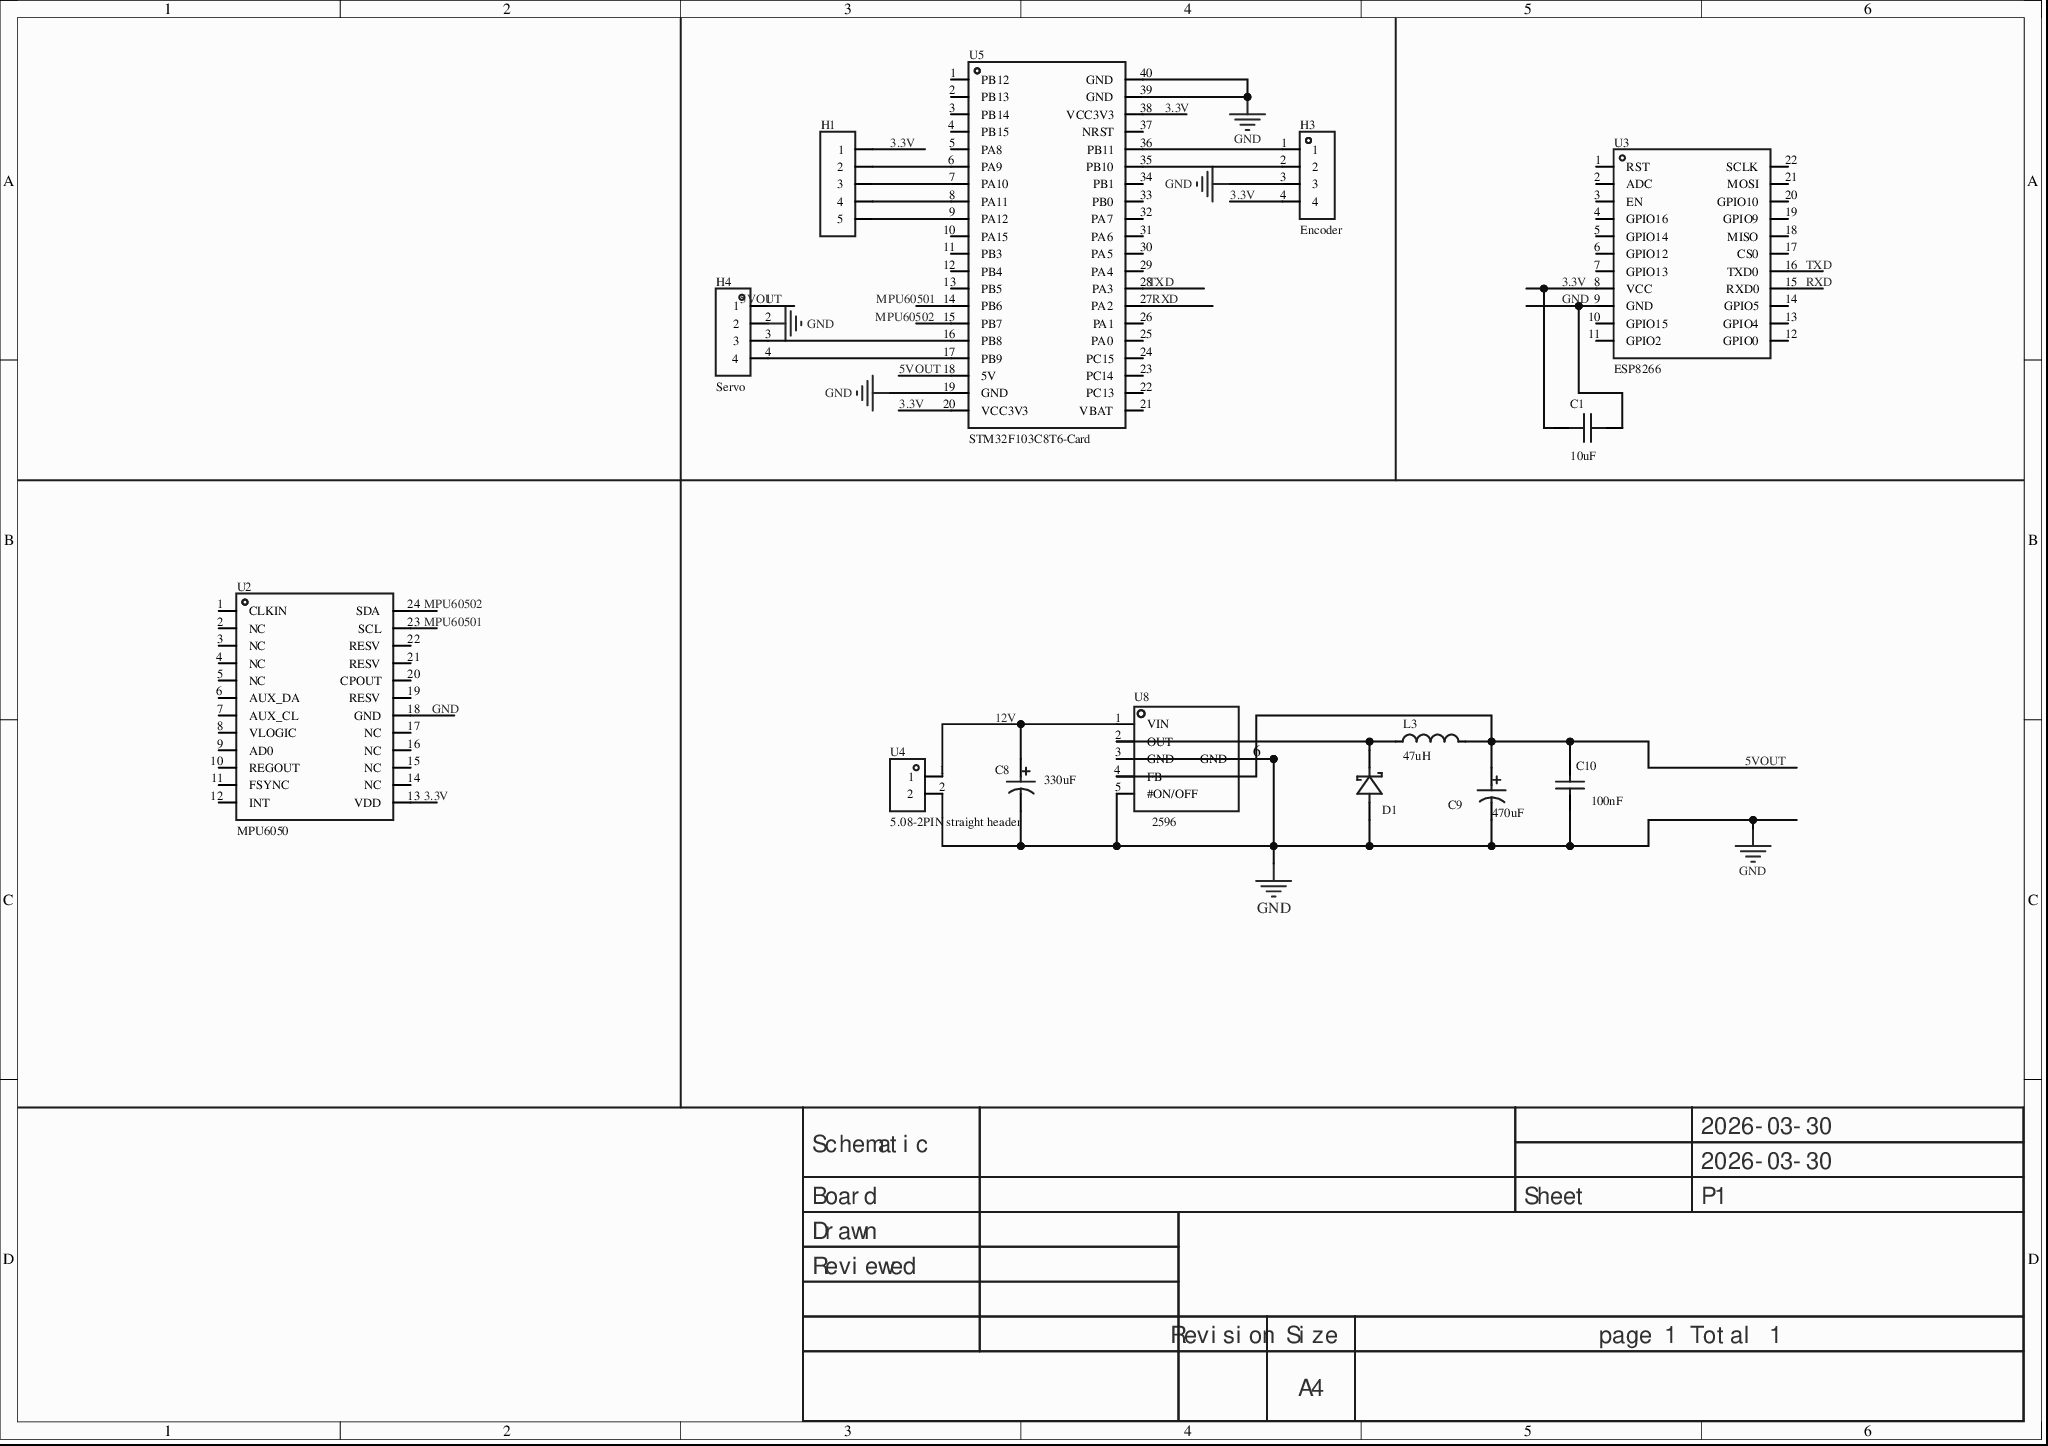
[diagram p0: MISC52071-3.schdoc]
# Altium project MISC52071-2.PrjPcb
1 sheet, 14 parts. Net scope: global (net labels, ports and power ports of the same name join across sheets).
Board file: MISC52071.pcbdoc

## Sheet MISC52071-3.schdoc
size 297 x 209 mm; Version: V1.0; @Project Name: MISC52071; @Update Date: 2026-03-30; @Create Date: 2026-03-30; @Board Name: MISC52071; @Create Time: 10:07:17; @Page Count: 1; @Page No: 1; @Schematic Name: MISC52071; @Update Time: 10:07:17; Size: A4

### Parts
C1  10uF  [C0603]
C8  value 330uF  [CAP-SMD_BD8.0-L8.3-W8.3-RD]
C9  value 470uF  [CAP-SMD_BD8.0-L8.3-W8.3-RD]
C10  value 100nF  [C0805]
D1  (no value)  [SMA_L4.3-W2.6-LS5.2-RD]
H1  (no value)  [HDR-TH_5P-P2.54-V-F]
H3  Encoder  [HDR-TH_4P-P2.54-V-M]
H4  Servo  [HDR-TH_4P-P2.54-V-M]
L3  value 47uH  [IND-SMD_L7.0-W6.6]
U2  MPU6050  [QFN-24_L4.0-W4.0-P0.50-BL]
U3  ESP8266  [WIFIM-SMD_ESP-12F-ESP8266MOD]
U4  5.08-2PIN straight header  [HDR-TH_2P-P5.08_C9900004333]
U5  STM32F103C8T6-Card  [CONN-TH_L53.3-W22.9_STM32F103C8T6-CARD]
U8  LM2596S-5.0  [TO-263-5_L10.2-W8.9-P1.70-BR]  (value not drawn)

### Nets
GND: C1.2 C8.2 C9.2 C10.2 D1.2(A) H3.3 H4.2 U2.18(GND) U3.9(GND) U4.2 U5.19(GND) U5.39(GND) U5.40(GND) U8.3(GND) U8.5(#ON/OFF) U8.6(GND)
3.3V: C1.1 H1.1 H3.4 U2.13(VDD) U3.8(VCC) U5.20(VCC3V3) U5.38(VCC3V3)
5VOUT: C9.1 C10.1 H4.1 L3.2 U5.18(5V) U8.4(FB)
12V: C8.1 U4.1 U8.1(VIN)
MPU60501: U2.23(SCL) U5.14(PB6)
MPU60502: U2.24(SDA) U5.15(PB7)
RXD: U3.15(RXD0) U5.27(PA2)
TXD: U3.16(TXD0) U5.28(PA3)
NetD1_1: D1.1(K) L3.1 U8.2(OUT)
NetH1_2: H1.2 U5.6(PA9)
NetH1_3: H1.3 U5.7(PA10)
NetH1_4: H1.4 U5.8(PA11)
NetH1_5: H1.5 U5.9(PA12)
NetH3_1: H3.1 U5.36(PB11)
NetH3_2: H3.2 U5.35(PB10)
NetH4_3: H4.3 U5.16(PB8)
NetH4_4: H4.4 U5.17(PB9)

Not connected (* = marked no-connect by the designer): U2 1(CLKIN) 2(NC) 3(NC) 4(NC) 5(NC) 6(AUX_DA) 7(AUX_CL) 8(VLOGIC) 9(AD0) 10(REGOUT) 11(FSYNC) 12(INT) 14(NC) 15(NC) 16(NC) 17(NC) 19(RESV) 20(CPOUT) 21(RESV) 22(RESV); U3 1(RST) 2(ADC) 3(EN) 4(GPIO16) 5(GPIO14) 6(GPIO12) 7(GPIO13) 10(GPIO15) 11(GPIO2) 12(GPIO0) 13(GPIO4) 14(GPIO5) 17(CS0) 18(MISO) 19(GPIO9) 20(GPIO10) 21(MOSI) 22(SCLK); U5 1(PB12) 2(PB13) 3(PB14) 4(PB15) 5(PA8) 10(PA15) 11(PB3) 12(PB4) 13(PB5) 21(VBAT) 22(PC13) 23(PC14) 24(PC15) 25(PA0) 26(PA1) 29(PA4) 30(PA5) 31(PA6) 32(PA7) 33(PB0) 34(PB1) 37(NRST)

### Notes on the sheet
- 2026-03-30
- Schematic
- Board
- Sheet
- P1
- Drawn
- Reviewed
- Revision
- Size
- A4
- page 1 Total 1

### Library data of the parts
C1 = CAP_0603: Symbol: Capacitance; ConvertToPcb: yes; ModelId: ac125912035d415993ca9572d50418b10819f05c4eef4c71ace90d822a990e87; ModelName: C0603_L1.6-W0.8-H0.8; ModelTransform: 62.992,31.496,0,0,0,0,0,0,0; Device: CAP_0603; Value: 10uF; AddInBom: yes; Supplier Footprint: 0603; FootprintName: C0603
C8 C9 = CS1V221M-CRF10　: Capacitance: 220uF; Tolerance: ±20%; Rated voltage: 35V; Body diameter: 8mm; Body length: 10.5mm; Ripple current: -; ESR: -; Lifetime: 2000hrs@105; Operating temperature: -40~+105;; Manufacturer: ST(先科); Rated Voltage: 25V; 3D Model: b102f1362be24624a1b1334fec8dc7f4; 3D Model Transform: 354.33,326.81037,0,0,0,0,0,0,0; AddInBom: yes; Symbol: CS1V221M-CRF10; Device: CS1V221M-CRF10; Lifetime @ Temp: 2000hrs@105; Operating Temperature: -40~+105; Manufacturer Part: CS1V221M-CRF10; Supplier Footprint: SMD,8x10.5mm; JLCPCB Part Class: Extended Part; Datasheet: https://atta.szlcsc.com/upload/public/pdf/source/20170325/1490427945143.pdf; Supplier: LCSC; φD: 8mm; L: 10.5mm; Ripple Current: -; Equivalent Series Resistance(ESR): -; ConvertToPcb: yes; FootprintName: CAP-SMD_BD8.0-L8.3-W8.3-RD; ModelName: CAP-SMD_BD8.0-L8.3-W8.3-RD
  C8: Supplier Part: C97814
C10 = CL21B104KBCNNNC: Capacitance: 100nF; Tolerance: ±10%; Rated voltage: 50V; Temperature coefficient: X7R;; Manufacturer: SAMSUNG(三星); 3D Model: 1ba041120af144c991958decab20d241; 3D Model Transform: 78.74,51.181,0,0,0,0,0,0.0005,0; AddInBom: yes; ModelName: C0805_L2.0-W1.3-H1.3; Symbol: CL21B104KBCNNNC; Device: CL21B104KBCNNNC; LCSC Part Name: 100nF ±10% 50V; Supplier Part: C1711; Manufacturer Part: CL21B104KBCNNNC; Supplier Footprint: 0805; JLCPCB Part Class: Extended Part; Datasheet: https://atta.szlcsc.com/upload/public/pdf/source/20160103/1457707693305.pdf; Supplier: LCSC; Voltage Rated: 50V; Temperature Coefficient: X7R; ConvertToPcb: yes; FootprintName: C0805
D1 = SS34_3: Manufacturer: TDD(台冠电子); Manufacturer Part: SS34; Symbol: SS34_C3032484; 3D Model: 7ed2c9d0a4a74bbdbba07ab4052caf5b; 3D Model Transform: 185.039,102.362,0,0,0,0,0,0,0; AddInBom: yes; Device: SS34_3; LCSC Part Name: SS34; Supplier Part: C3032484; Supplier Footprint: SMA; JLCPCB Part Class: Extended Part; Datasheet: https://atta.szlcsc.com/upload/public/pdf/source/20220622/9D70D0693761B542BF6F533590093AA5.pdf; Supplier: LCSC; ConvertToPcb: yes; FootprintName: SMA_L4.3-W2.6-LS5.2-RD; ModelName: SMA_L4.3-W2.6-LS5.2-RD
H1 = HDR-F_2.54_1x5P: Symbol: Header-Female-2.54_1x5; ConvertToPcb: yes; ModelId: f49cb6116a3d45e5a64915bf3e00773f0819f05c4eef4c71ace90d822a990e87; ModelTransform: 519.684,98.464,0,0,0,0,0,0,-124.016; Device: HDR-F_2.54_1x5P; AddInBom: yes; SupplierPart: C50950; Supplier Footprint: 插件; FootprintName: HDR-TH_5P-P2.54-V-F; ModelName: HDR-TH_5P-P2.54-V-F
H3 = PZ254V-11-04P: Pin structure: 1x4P; Pitch: 2.54mm; Row spacing: -; Square/round pins: Square; Mounting: Through-hole; Rows: Single row; Total pins: 4P; Rated current: 3A; Rated voltage: 250V; Mating pin length: 6mm; Housing height: 2.5mm; Tail length: 3mm; Contact material: -; Operating temperature: -40℃~+105℃; Color: Black;; Manufacturer Part: 编码器; Manufacturer: XFCN(兴飞); Symbol: PZ254V-11-04P_C2691448; 3D Model: 112f4d05e8d64e99ab9a333894bea4f90819f05c4eef4c71ace90d822a990e87; 3D Model Transform: 399.999,104.7242,0,0,0,0,0,0,-118.11; AddInBom: yes; ModelName: HDR-TH_4P-P2.54-M-LI-1X4P; Device: PZ254V-11-04P; LCSC Part Name: 1x4P 间距:2.54mm 方针 直插; Supplier Part: C2691448; Supplier Footprint: 插件,P=2.54mm; JLCPCB Part Class: Extended Part; Datasheet: https://item.szlcsc.com/datasheet/PZ254V-11-04P/2801085.html; Supplier: LCSC; Pin Structure: 1x4P; Row Spacing: -; Circluar Pins/Square Pins: Square; Mounting Type: Through-hole; Number of Rows: Single row; Number of Pins: 4P; Current Rating: 3A; Voltage Rating (Max): 250V; Length of Mating Pin: 6mm; Insulation Height: 2.5mm; Length of End Connection Pin: 3mm; Contact Material: -; Operating Temperature: -40℃~+105℃; Color: Black; ConvertToPcb: yes; FootprintName: HDR-TH_4P-P2.54-V-M
H4 = PZ254V-11-04P: Pin structure: 1x4P; Pitch: 2.54mm; Row spacing: -; Square/round pins: Square; Mounting: Through-hole; Rows: Single row; Total pins: 4P; Rated current: 3A; Rated voltage: 250V; Mating pin length: 6mm; Housing height: 2.5mm; Tail length: 3mm; Contact material: -; Operating temperature: -40℃~+105℃; Color: Black;; Manufacturer Part: 舵机; Manufacturer: XFCN(兴飞); Symbol: PZ254V-11-04P_C2691448; 3D Model: 112f4d05e8d64e99ab9a333894bea4f90819f05c4eef4c71ace90d822a990e87; 3D Model Transform: 399.999,104.7242,0,0,0,0,0,0,-118.11; AddInBom: yes; ModelName: HDR-TH_4P-P2.54-M-LI-1X4P; Device: PZ254V-11-04P; LCSC Part Name: 1x4P 间距:2.54mm 方针 直插; Supplier Part: C2691448; Supplier Footprint: 插件,P=2.54mm; JLCPCB Part Class: Extended Part; Datasheet: https://item.szlcsc.com/datasheet/PZ254V-11-04P/2801085.html; Supplier: LCSC; Pin Structure: 1x4P; Row Spacing: -; Circluar Pins/Square Pins: Square; Mounting Type: Through-hole; Number of Rows: Single row; Number of Pins: 4P; Current Rating: 3A; Voltage Rating (Max): 250V; Length of Mating Pin: 6mm; Insulation Height: 2.5mm; Length of End Connection Pin: 3mm; Contact Material: -; Operating Temperature: -40℃~+105℃; Color: Black; ConvertToPcb: yes; FootprintName: HDR-TH_4P-P2.54-V-M
L3 = CMLO0630H330MTT: Inductance: 33uH; Tolerance: ±20%; DCR: 270mΩ;; Manufacturer: Cybermax(思博科技); 3D Model: 6860c29aec394a38a0f014af7f722a42; 3D Model Transform: 275.6,259.8,0,0,0,0,0,0,0; AddInBom: yes; ModelName: IND-SMD_L7.0-W6.6-H3.0; Symbol: CMLO0630H330MTT; Device: CMLO0630H330MTT; LCSC Part Name: 33uH ±20% 270mΩ; Manufacturer Part: CMLO0630H330MTT; Supplier Footprint: SMD; JLCPCB Part Class: Extended Part; Datasheet: https://atta.szlcsc.com/upload/public/pdf/source/20201124/C961478_55C23F293F63DC1D2CF3D7AB16D0E182.pdf; Supplier: LCSC; DC Resistance (DCR): 270mΩ; ConvertToPcb: yes; FootprintName: IND-SMD_L7.0-W6.6
U2 = MPU6050: Symbol: MPU6050_C9900042518; AddInBom: yes; Device: MPU6050; LCSC Part Name: MPU6050; SupplierPart: C9900042518; ManufacturerPart: MPU6050; Supplier Footprint: QFN-24_L4.0-W4.0-P0.50-BL-EP2.7; Supplier: LCSC; ConvertToPcb: yes; FootprintName: QFN-24_L4.0-W4.0-P0.50-BL
U3 = ESP8266: AddInBom: yes; ModelId: c53b8c57aa74447bb5071c1a48f7c2190819f05c4eef4c71ace90d822a990e87; ModelName: WIFIM-SMD_WIFI-L24.0-W16.0-H3.1; ModelTransform: 630.707,945.274,0,90,0,0,-162.403,0,0; Symbol: ESP8266; Device: ESP8266; LCSC Part Name: ESP8266; SupplierPart: C9900003049; ManufacturerPart: ESP8266; Supplier Footprint: WIFIM-SMD; JLCPCB Part Class: Extended Part; Supplier: LCSC; ConvertToPcb: yes; FootprintName: WIFIM-SMD_ESP-12F-ESP8266MOD
U4 = 5.08-2PIN直针座: 3D Model: 91ee0a7c4b69475886d36596bbdbca0c0819f05c4eef4c71ace90d822a990e87; 3D Model Transform: 299.9994,98.425,0,0,0,0,0,0,-118.11; AddInBom: yes; Symbol: 5.08-2PIN straight header; Device: 5.08-2PIN straight header; LCSC Part Name: 5.08-2PIN直针座; Supplier Part: C9900004333; Manufacturer Part: 5.08-2PIN直针座; Supplier Footprint: 5.08-2PIN; JLCPCB Part Class: Extended Part; Supplier: LCSC; ConvertToPcb: yes; FootprintName: HDR-TH_2P-P5.08_C9900004333; ModelName: HDR-TH_2P-P5.08_C9900004333
U5 = STM32F103C8T6-Card: AddInBom: yes; Symbol: STM32F103C8T6-CARD; Device: STM32F103C8T6-Card; LCSC Part Name: STM32F103C8T6-Card; SupplierPart: C9900077949; ManufacturerPart: STM32F103C8T6-Card; Supplier Footprint: 插件; JLCPCB Part Class: Extended Part; Supplier: LCSC; ConvertToPcb: yes; FootprintName: CONN-TH_L53.3-W22.9_STM32F103C8T6-CARD
U8 = LM2596S-5.0_C347421: Function type: Step-down; Output type: Fixed; Input voltage: 40V; Output voltage: 5V; Output current (max): 3A;; Manufacturer: UMW(广东友台半导体); Symbol: LM2596-TO263; Add into BOM: yes; 3D Model: 4e421a816a7f4d57b8710832ddea550a; 3D Model Transform: 401.574,560.17797,0,90,0,0,-45.276,0,0; Synchronous Rectification: No; Number of Outputs: 1; Topology: Buck; Switching Frequency: 150kHz; ModelName: TO-263-5-5P_L10.2-W8.7-H4.5-LS14.4-P1.70; Device: LM2596S-5.0_C347421; Convert to PCB: yes; LCSC Part Name: 降压型 输入40V 输出5V 3A; Supplier Part: C347421; Manufacturer Part: LM2596S-5.0; Supplier Footprint: TO-263-5; JLCPCB Part Class: Extended Part; Datasheet: https://atta.szlcsc.com/upload/public/pdf/source/20211011/C7416AEF3194BD283261B8F2553C4145.pdf; Supplier: LCSC; Function: Step-down; Output Type: Fixed; Input Voltage: 40V; Output Voltage: 5V; Output Current (Max): 3A; Operating Temperature: -40℃~+125℃@(TA); FootprintName: TO-263-5_L10.2-W8.9-P1.70-BR